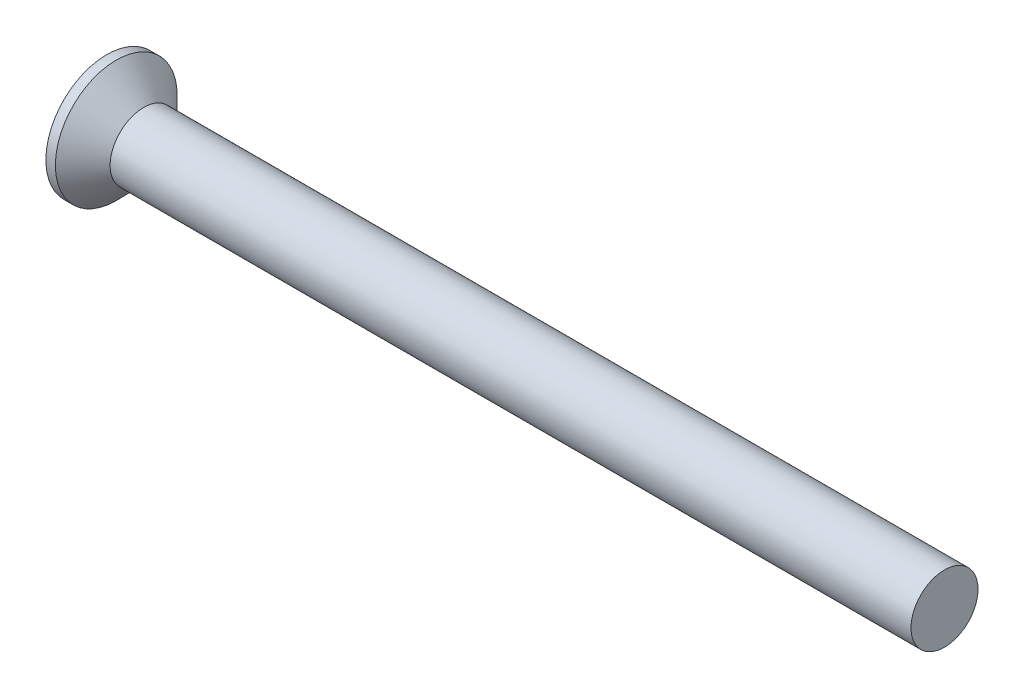
SolidWorks part; units mm, degrees
ref_plane "Front" through (0, 0, 0) normal (0, 0, 1) x (1, 0, 0)
ref_plane "Top" through (0, 0, 0) normal (0, 1, 0) x (1, 0, 0)
ref_plane "Right" through (0, 0, 0) normal (1, 0, 0) x (0, 0, -1)
sketch "Sketch1" plane through (0, 0, 0) normal (0, 0, 1) x (1, 0, 0)
  line L0 (75, 3) -> (5.3, 3)
  line L1 (5.3, 3) -> (3.3, 3)
  line L2 (3.3, 3) -> (0.85, 5.45)
  line L3 (0.85, 5.45) -> (0, 5.45)
  line L4 (75, 3) -> (75, 0)
  line L5 (4.5158, 0) -> (-89.8219, 0) construction
  line L6 (75, 0) -> (0, 0)
  line L7 (0, 5.45) -> (0, 0)
revolve "Base" add sketch "Sketch1" angle 360 about L5
cosmetic thread "ThreadCosmetic1" [suppressed] parameters "bb"=56.7, "THD_MINOR"=4.917
sketch "Sketch6" plane through (0, 0, 0) normal (1, 0, 0) x (0, 0, -1)
  line L0 (-1.9271, 0) -> (2.0512, 0) construction
  line L1 (0, 1.8651) -> (0, -2.0207) construction
  line L2 (0.68, 0.68) -> (0.68, 3.4)
  line L3 (0.68, 3.4) -> (-0.68, 3.4)
  line L4 (-0.68, 0.68) -> (-0.68, 3.4)
  line L5 (0.68, 0.68) -> (3.4, 0.68)
  line L6 (3.4, 0.68) -> (3.4, -0.68)
  line L7 (-3.4, 0.68) -> (-3.4, -0.68)
  line L8 (-0.68, 0.68) -> (-3.4, 0.68)
  line L9 (-0.68, -0.68) -> (-3.4, -0.68)
  line L10 (0.68, -0.68) -> (3.4, -0.68)
  line L11 (-0.68, -0.68) -> (-0.68, -3.4)
  line L12 (0.68, -3.4) -> (-0.68, -3.4)
  line L13 (0.68, -0.68) -> (0.68, -3.4)
  point P16 (-3.4, 0)
  point P17 (3.4, 0)
extrude "CrossRecess" cut sketch "Sketch6" along normal blind 1.65
draft "Draft9" type of draft neutral plane draft angle 30 faces to draft 4 face at (0.825, -3.4, 0) face at (0.825, 0, 3.4) face at (0.825, 0, -3.4) face at (0.825, 3.4, 0) neutral plane through (0, 5.45, 0) neutral plane normal (-1, 0, 0) parameters "D1"=30
fillet "Fillet5" radius 0.3 4 edges at (0.825, -0.68, -0.68) (0.825, -0.68, 0.68) (0.825, 0.68, -0.68) (0.825, 0.68, 0.68)
sketch "Sketch7" plane through (0, 0, 0) normal (1, 0, 0) x (0, 0, -1)
  line L0 (-2.0126, 0) -> (1.9757, 0) construction
  line L1 (0, 1.9314) -> (0, -2.0126) construction
  line L2 (0, 0) -> (1.5555, 1.5555) construction
  line L3 (0, 1.0161) -> (2.4042, 2.4042)
  line L4 (-1.5402, 1.5402) -> (0, 0) construction
  line L5 (1.0161, 0) -> (2.4042, 2.4042)
  line L6 (0, -1.0161) -> (2.4042, -2.4042)
  line L7 (1.0161, 0) -> (2.4042, -2.4042)
  line L8 (-1.0161, 0) -> (-2.4042, -2.4042)
  line L9 (0, -1.0161) -> (-2.4042, -2.4042)
  line L10 (-1.0161, 0) -> (-2.4042, 2.4042)
  line L11 (0, 1.0161) -> (-2.4042, 2.4042)
  dimension "D3" = 15
extrude "Cut-Extrude3" [suppressed] cut sketch "Sketch7" along normal blind 10 draft 20
sketch "Sketch10" plane through (0, 0, 0) normal (0, 0, 1) x (1, 0, 0)
  line L0 (62.2289, 0) -> (-1.9277, 0) construction
  line L1 (3.3, 3) -> (4.3, 3)
  line L4 (4.3, 3) -> (4.3, 0)
  line L7 (4.3, 0) -> (3.3, 0)
  line L9 (3.3, 3) -> (0.85, 5.45) construction
  line L10 (3.3, 3) -> (3.3, 0)
  dimension "p" = 1
revolve "Revolve2" add sketch "Sketch10" angle 360 about L0
sketch "Sketch8" plane through (0, 0, 0) normal (0, 0, 1) x (1, 0, 0)
  line L0 (37, 3) -> (34.5, 2.4585)
  line L1 (34.5, 2.4585) -> (5, 2.4585)
  line L3 (75, -3) -> (75, 3) construction
  line L6 (5, 2.4585) -> (5, 7.4585)
  line L7 (5, 7.4585) -> (37, 7.4585)
  line L8 (37, 7.4585) -> (37, 3)
  line L9 (62.4753, 0) -> (52.9594, 0) construction
  dimension "D1" = 5
  dimension "x" = 2.5
sketch "Sketch11" plane through (0, 0, 0) normal (0, 0, 1) x (1, 0, 0)
  line L0 (75, 2.531) -> (75.2707, 3)
  line L1 (75.2707, 3) -> (75.2707, 3.5415)
  line L2 (75.2707, 3.5415) -> (74.7292, 3.5415)
  line L3 (74.7292, 3.5415) -> (74.7292, 3)
  line L4 (74.7292, 3) -> (75, 2.531)
  line L5 (75, -3) -> (75, 3) construction
  line L6 (0, 0) -> (66.0064, 0) construction
revolve "Cut-Revolve10" [suppressed] cut sketch "Sketch11" angle 360 about L6
pattern_linear "LPattern10" [suppressed] count 87 spacing 0.6498 along (1, 0, 0)
equation "\"D1@Sketch6\" = \"m@Sketch6\" / 5"
equation "\"D1@CrossRecess\" = \"k@Sketch1\" / 2"
equation "\"D1@Sketch11\" = \"d@Sketch1\""
equation "\"D2@Sketch11\" =  ( \"d@Sketch1\" - \"THD_MINOR@ThreadCosmetic1\" )  / 2"
equation "\"D3@LPattern10\" = \"D2@Sketch11\" * 1.2"
equation "\"D1@LPattern10\" = \"bb@ThreadCosmetic1\" / \"D3@LPattern10\" "
